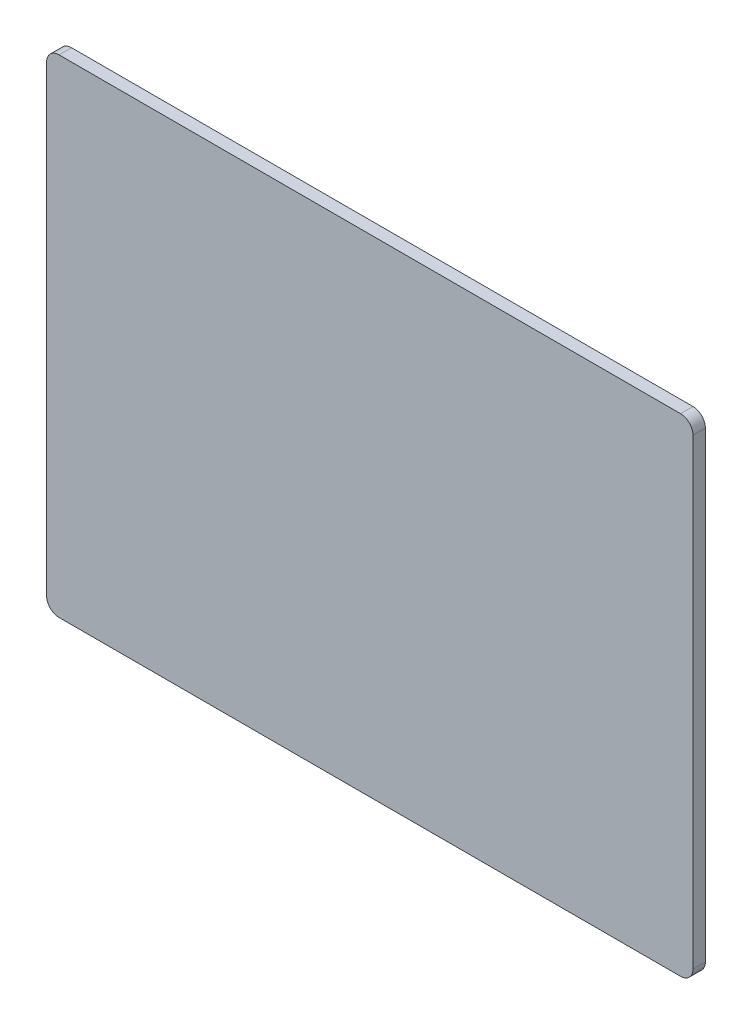
SolidWorks part; units mm, degrees
material "Plain Carbon Steel"
ref_plane "Front Plane" through (0, 0, 0) normal (0, 0, 1) x (1, 0, 0)
ref_plane "Top Plane" through (0, 0, 0) normal (0, 1, 0) x (1, 0, 0)
ref_plane "Right Plane" through (0, 0, 0) normal (1, 0, 0) x (0, 0, -1)
sketch "Sketch1" plane through (0, 0, 0) normal (0, 0, 1) x (1, 0, 0)
  line L1 (0, 0) -> (260, 0)
  line L2 (0, 0) -> (0, -196)
  line L3 (0, -196) -> (260, -196)
  line L4 (260, 0) -> (260, -196)
  dimension "D1" = 260
  dimension "D2" = 196
extrude "Boss-Extrude1" add sketch "Sketch1" along normal blind 5
fillet "Fillet1" radius 5 4 edges at (260, 0, 2.5) (260, -196, 2.5) (0, -196, 2.5) (0, 0, 2.5)
